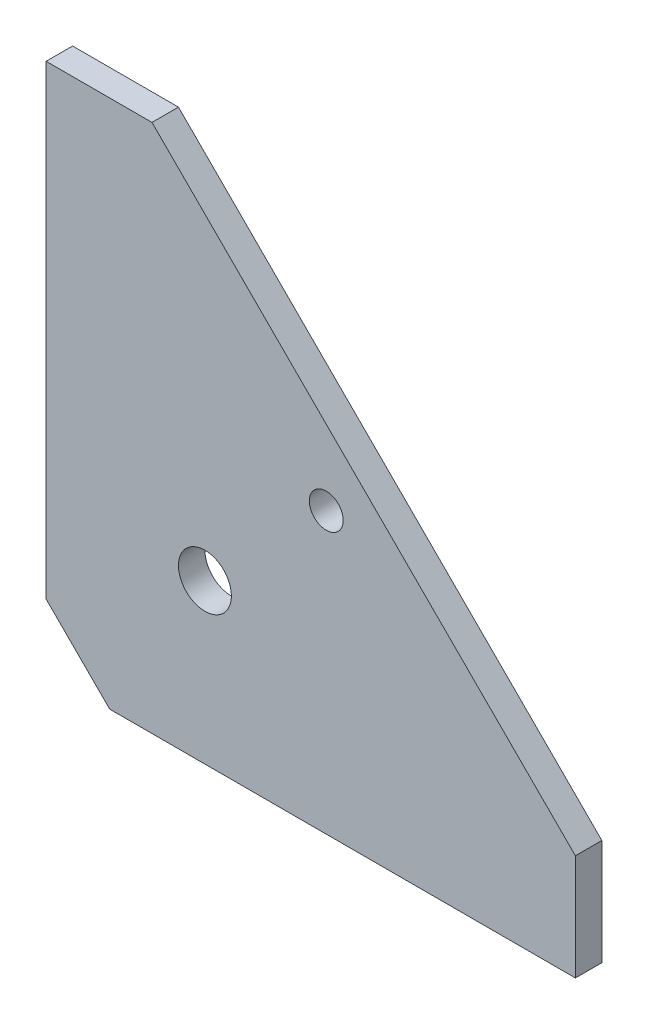
from build123d import *

# Parameters (mm, degrees)
BOSS_EXTRUDE1_DEPTH = 25
SKETCH2_R           = 25
CUT_EXTRUDE1_DEPTH  = 25
CHAMFER1_SIZE       = 60
SKETCH3_R           = 16
CUT_EXTRUDE2_DEPTH  = 708.548584904


with BuildPart() as part:
    # Sketch1 → Boss-Extrude1 (new body)
    with BuildSketch(Plane.XY):
        Polygon((0, 0), (0, 500), (100, 500), (500, 100), (500, 0), align=None)
    extrude(amount=BOSS_EXTRUDE1_DEPTH)

    # Sketch2 → Cut-Extrude1 (cut)
    with BuildSketch(Plane.XY.offset(25)):
        with Locations((150, 150)):
            Circle(SKETCH2_R)
    extrude(amount=-CUT_EXTRUDE1_DEPTH, mode=Mode.SUBTRACT)

    # Chamfer1
    chamfer1_edges = [part.edges().sort_by_distance(p)[0] for p in [
        (0, 0, 12.5),
    ]]
    chamfer(chamfer1_edges, length=CHAMFER1_SIZE)

    # Sketch3 → Cut-Extrude2 (cut, through all)
    with BuildSketch(Plane.XY.offset(25)):
        with Locations((264.644660941, 264.644660941)):
            Circle(SKETCH3_R)
    extrude(amount=-CUT_EXTRUDE2_DEPTH, mode=Mode.SUBTRACT)


solid = part.part
